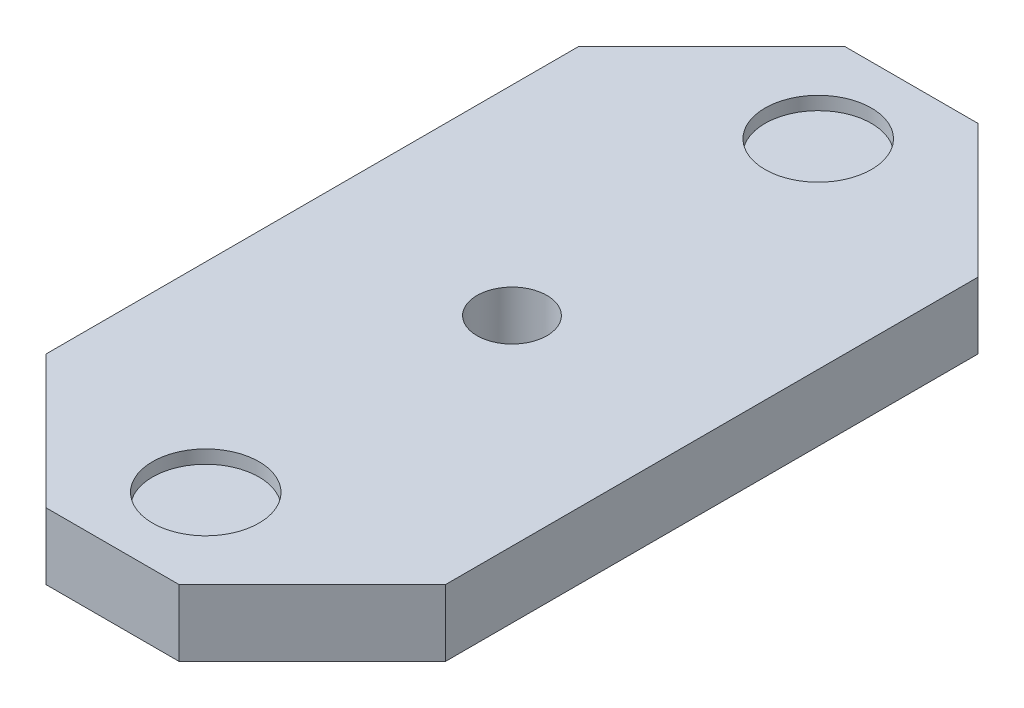
from build123d import *

# Parameters (mm, degrees)
SKETCH_1_W          = 60
SKETCH_1_H          = 120
EXTRUDE_1_DEPTH     = 10
SKETCH_2_R          = 8
CUT_EXTRUDE_1_DEPTH = 2
CHAMFER_1_SIZE      = 20
CUT_EXTRUDE_2_REACH = 69.823
SKETCH_3_R          = 5.25


with BuildPart() as part:
    # 草图1 → 凸台-拉伸1 (new body)
    with BuildSketch(Plane(origin=(0, 0, 0), x_dir=(1, 0, 0), z_dir=(0, 1, 0))):
        Rectangle(SKETCH_1_W, SKETCH_1_H)
    extrude(amount=EXTRUDE_1_DEPTH)

    # 草图2 → 切除-拉伸1 (cut)
    with BuildSketch(Plane(origin=(0, 10, 0), x_dir=(1, 0, 0), z_dir=(0, 1, 0))):
        with Locations(Location((0, 46, 0), (0, 0, 270))):
            Circle(SKETCH_2_R)
        with Locations(Location((0, -46, 0), (0, 0, 270))):
            Circle(SKETCH_2_R)
    extrude(amount=-CUT_EXTRUDE_1_DEPTH, mode=Mode.SUBTRACT)

    # 倒角1
    chamfer_1_edges = [part.edges().sort_by_distance(p)[0] for p in [
        (30, 5, 60),
        (-30, 5, 60),
        (-30, 5, -60),
        (30, 5, -60),
    ]]
    chamfer(chamfer_1_edges, length=CHAMFER_1_SIZE)

    # 草图3 → 切除-拉伸2 (cut, up to next)
    with BuildSketch(Plane(origin=(0, 10, 0), x_dir=(1, 0, 0), z_dir=(0, 1, 0)), mode=Mode.PRIVATE) as cut_extrude_2_sk1:
        with Locations(Location((0, 0, 0), (0, 0, 270))):
            Circle(SKETCH_3_R)
    cut_extrude_2_tool1 = extrude(cut_extrude_2_sk1.sketch, amount=-CUT_EXTRUDE_2_REACH, mode=Mode.PRIVATE) & part.part
    add(cut_extrude_2_tool1.solids().sort_by_distance((0, 10, 0))[0], mode=Mode.SUBTRACT)


solid = part.part
